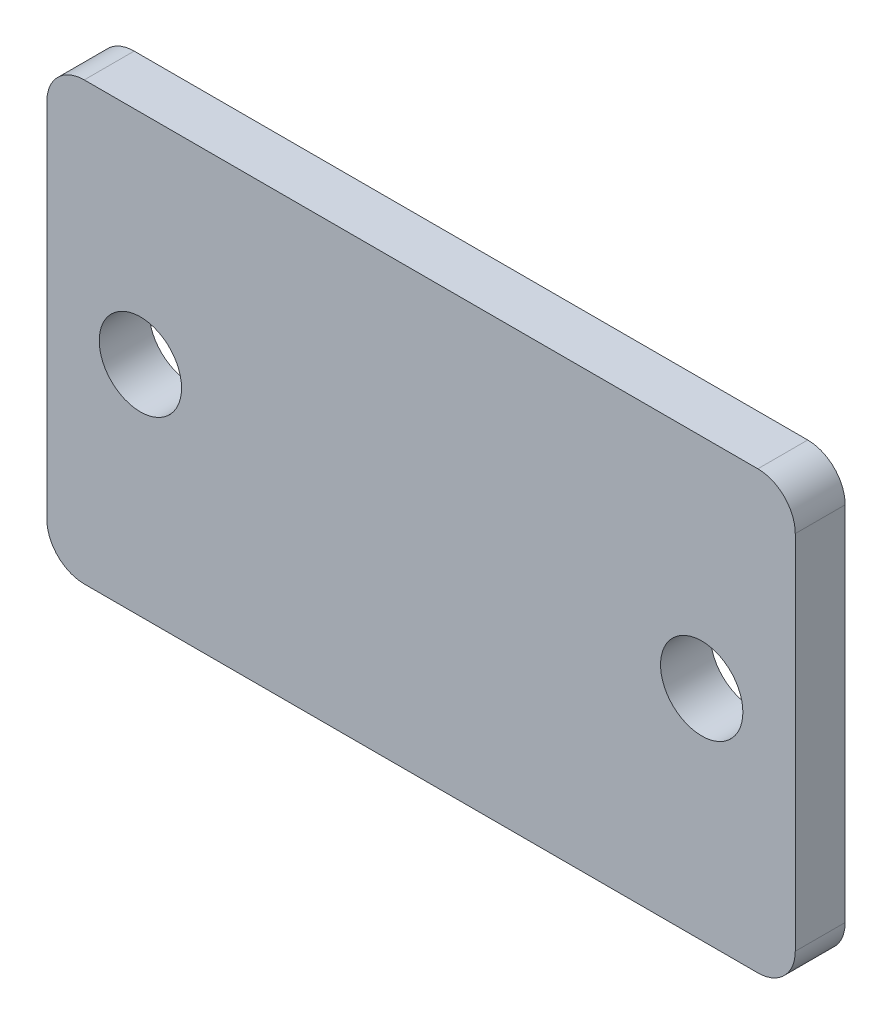
from build123d import *

# Parameters (mm, degrees)
SKETCH_1_W      = 60
SKETCH_1_H      = 35
SKETCH_1_R      = 3.3
EXTRUDE_1_DEPTH = 4
FILLET_1_R      = 3


with BuildPart() as part:
    # 草图1 → 凸台-拉伸1 (new body)
    with BuildSketch(Plane.XY):
        Rectangle(SKETCH_1_W, SKETCH_1_H)
        with Locations((-22.5, 0)):
            Circle(SKETCH_1_R, mode=Mode.SUBTRACT)
        with Locations((22.5, 0)):
            Circle(SKETCH_1_R, mode=Mode.SUBTRACT)
    extrude(amount=EXTRUDE_1_DEPTH)

    # 圆角1
    fillet_1_edges = [part.edges().sort_by_distance(p)[0] for p in [
        (30, -17.5, 2),
        (-30, -17.5, 2),
        (-30, 17.5, 2),
        (30, 17.5, 2),
    ]]
    fillet(fillet_1_edges, radius=FILLET_1_R)


solid = part.part
